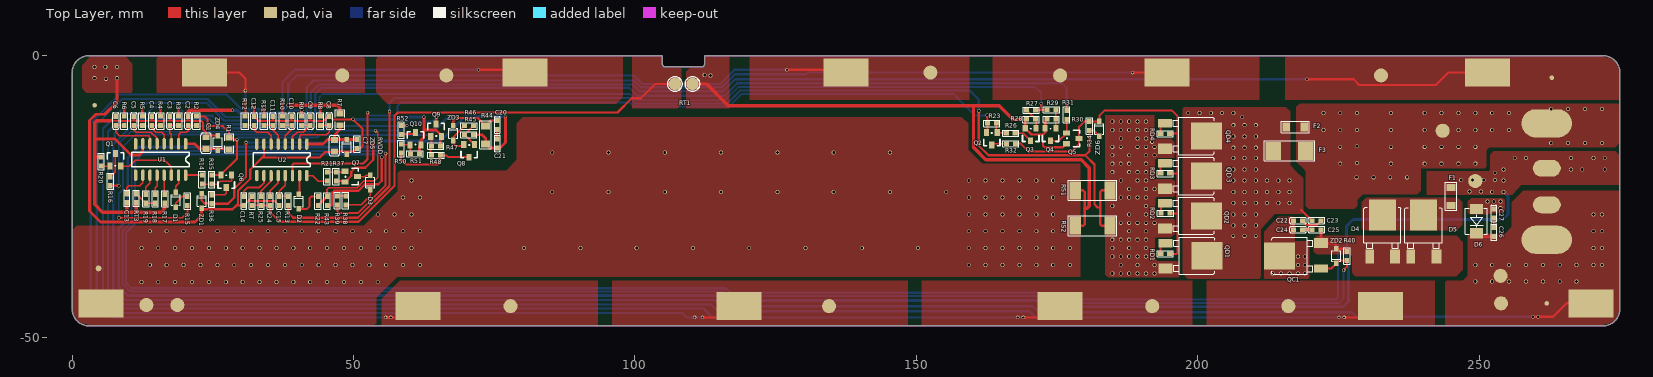
[diagram p0: Top Layer view]
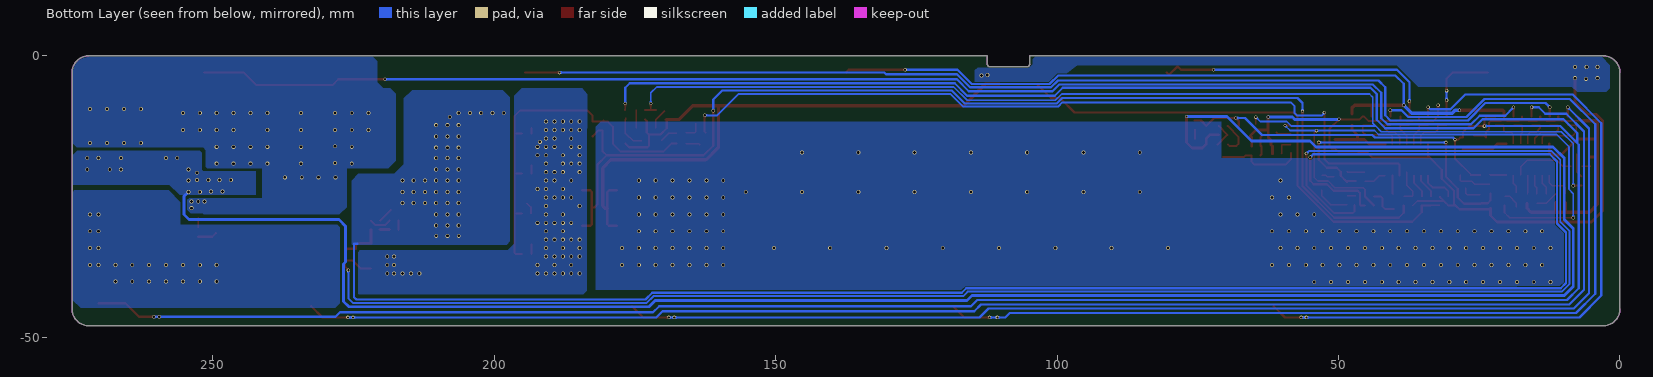
[diagram p1: Bottom Layer view, seen from below]
# Altium PCB MISC86331.PcbDoc
Units mm, origin at the board's own origin, x right, y up, seen from the top; angles counter-clockwise.
Board outline 275 x 48 mm, 2 copper layers (Top Layer, Bottom Layer); 113 components, 80 nets, 305 pads, 410 vias.

## Layer stack, top to bottom (the 12.6 mil dielectric is the usual default, probably not edited)
Top Solder: solder mask 0.0102, Solder Resist, Dk 3.5
Top Layer: signal copper 0.0356
Dielectric 1: dielectric 0.32, FR-4, Dk 4.8
Bottom Layer: signal copper 0.0356
Bottom Solder: solder mask 0.0102, Solder Resist, Dk 3.5

## Board outline
0,-45 0,-3 cw(c3,-3) 3,0 104.875,0 104.875,-1.5 ccw(c105.375,-1.5) 105.375,-2 111.875,-2 ccw(c111.875,-1.5) 112.375,-1.5 112.375,0 272,0 cw(c272,-3) 275,-3 275,-45 cw(c272,-45) 272,-48 3,-48 cw(c3,-45)

## Design rules (kind name [scope] priority, off if disabled: settings)
Clearance "Stitching CS" [IsStitchingVia and InNet('CS') vs (IsVia and (Not IsStitchingVia)) Or IsPad] p1: gap=0.127 ignorepadtopadclearanceinfootprint=FALSE
Clearance [All] p2: gap=0.2 ignorepadtopadclearanceinfootprint=FALSE
ComponentClearance [All] p1: gap=0.2 collisioncheckmode=3 verticalgap=0.254 showdistances=FALSE
PolygonConnect [All] p1: connectstyle=Direct reliefconductorwidth=0.254 reliefentries=4 polygonreliefangle="90 Angle" airgapwidth=0.254
RoutingVias [All] p1: holewidth=0.4 width=0.6 viastyle="Through Hole" minholewidth=0.4 minwidth=0.6 maxholewidth=0.4 maxwidth=0.6
SolderMaskExpansion [All] p1: expansion=0.102 istentingtop=FALSE
Width [All] p1: maxlimit=1 minlimit=0.2 preferedwidth=0.25
29 further rules are at their usual default settings.

## Components (designator, comment, footprint, x,y, rotation, side; value= is the part's Value field where it differs from the comment)
C1 "1uF" CAP0805 23.8,-15.517 r90 top
C2 "0.1uF" C0603A 20.601,-11.58 r180 top
C3 "0.1uF" C0603A 17.388,-11.58 r180 top
C4 "0.1uF" C0603A 14.175,-11.58 r180 top
C5 "0.1uF" C0603A 10.963,-11.58 r180 top
C6 "0.1uF" C0603A 7.75,-11.58 r180 top
C7 "1uF" CAP0805 46.6,-16.016 r270 top
C8 "0.1uF" C0603A 45.68,-11.58 r180 top
C9 "0.1uF" C0603A 42.341,-11.58 r180 top
C10 "0.1uF" C0603A 39.003,-11.58 r180 top
C11 "0.1uF" C0603A 35.665,-11.58 r180 top
C12 "0.1uF" C0603A 32.327,-11.58 r180 top
C13 "0.1uF" C0603A 9.718,-25.324 r0 top
C14 "0.1uF" C0603A 30.5,-25.8 r0 top
C15 "0.1uF" C0603A 36.8,-25.8 r180 top
C20 "0.1uf" C0603A 75.535,-12.323 r0 top
C21 "0.1uf" C0603A 75.535,-15.598 r0 top
C22 "0.1uF" C0603A 217.8,-29.3 r270 top
C23 "0.1uF" C0603A 221.1,-29.3 r90 top
C24 "0.1uF" C0603A 217.8,-30.9 r270 top
C25 "0.1uF" C0603A 221.1,-30.9 r270 top
C26 "0.1uF" C0603A 252.583,-31.354 r0 top
C27 "0.1uF" C0603A 252.583,-28.016 r0 top
D1 "1N4148" SOD323 18.4,-25.608 r90 top
D2 "1N4148" SOD323 40.3,-25.902 r90 top
D3 "1N4148" SOD323 53.016,-22.516 r270 top
D4 "SS510" TO-252-A 230.586,-35.481 r0 top
D5 "SS510" TO-252-A 237.9,-35.5 r0 top
D6 "RS2M" SMB-1 249.483,-29.379 r90 top
F1 "5A" R1206 245,-25 r90 top
F2 "30A" R1206 217.322,-12.65 r0 top
F3 "NC" 2410 213.396,-16.926 r0 top
Q1 "MMBT5401" SOT-23-3 7.7,-18.5 r0 top
Q2 "BSS84" SOT-23-3 163.409,-14.767 r180 top
Q3 "MMBT5551" SOT-23-3 170.31,-14.01 r180 top
Q4 "MMBT5551" SOT-23-3 173.836,-14.01 r180 top
Q5 "MMBT5551" SOT-23-3 177.8,-14.7 r270 top
Q6 "MMBT5401" SOT-23-3 27.4,-22.303 r180 top
Q7 "MMBT5401" SOT-23-3 49.616,-21.472 r270 top
Q8 "MMBT5401" SOT-23-3 70.547,-16.907 r180 top
Q9 "MMBT5551" SOT-23-3 64.668,-13.237 r0 top
Q10 "MMBT5551" SOT-23-3 61.017,-14.746 r0 top
QC1 "NMOS" TO-252-A 221.711,-37.784 r90 top
QD1 "NMOS" TO-252-A 194.467,-33.327 r270 top
QD2 "NMOS" TO-252-A 194.387,-26.237 r270 top
QD3 "NMOS" TO-252-A 194.387,-19.147 r270 top
QD4 "NMOS" TO-252-A 194.387,-12.058 r270 top
R1 "1K" RES0805 27.9,-14.568 r270 top
R2 "1K" RES0603 22.119,-11.581 r0 top
R3 "1K" RES0603 18.906,-11.581 r0 top
R4 "1K" RES0603 15.693,-11.581 r0 top
R5 "1K" RES0603 12.481,-11.581 r0 top
R6 "1K" RES0603 9.268,-11.581 r0 top
R7 "1K" RES0805 47.6,-10.313 r270 top
R8 "1K" RES0603 44.099,-11.581 r0 top
R9 "1K" RES0603 40.761,-11.581 r0 top
R10 "1K" RES0603 37.423,-11.581 r0 top
R11 "1K" RES0603 34.084,-11.581 r180 top
R12 "1K" RES0603 30.746,-11.581 r0 top
R13 "1K" R0603A 38.4,-25.8 r0 top
R14 "5.1M" R0603A 23.1,-22 r0 top
R15 "51K" R0603A 20.5,-25.8 r0 top
R16 "5.1M" R0603A 6.8,-22.3 r180 top
R17 "1K" R0603A 16.505,-25.416 r0 top
R18 "22K" R0603A 14.78,-25.416 r0 top
R19 "35K" R0603A 13.13,-25.416 r0 top
R20 "2M" R0603A 5.2,-18.8 r0 top
R21 "5.1M" R0603A 45.316,-21.472 r180 top
R22 "100K" R0603A 43.7,-25.8 r0 top
R23 "2M" R0603A 163.409,-12.039 r90 top
R24 "22K" R0603A 35.2,-25.8 r0 top
R25 "35K" R0603A 33.6,-25.8 r0 top
R26 "1M" R0603A 166.772,-13.764 r90 top
R27 "1M" R0603A 170.4,-9.7 r90 top
R28 "1M" R0603A 170.38,-11.326 r90 top
R29 "1M" R0603A 174.007,-9.614 r90 top
R30 "1M" R0603A 173.98,-11.326 r90 top
R31 "2M" R0603A 176.7,-10.5 r180 top
R32 "1K" R0603A 166.78,-15.626 r270 top
R34 "5.1M" R0603A 180.75,-12.5 r180 top
R35 "1M" R0603A 24.8,-22 r180 top
R36 "2M" R0603A 24.8,-25.5 r0 top
R37 "1M" R0603A 46.916,-21.472 r0 top
R38 "1M" R0603A 48.6,-25.75 r180 top
R39 "1M" R0603A 47.125,-25.75 r180 top
R40 "3M" R0603A 226.5,-35.6 r0 top
R43 "100K" R0603A 45.3,-25.8 r180 top
R44 "47K/1206" R1206 73.485,-14.073 r90 top
R45 "1M" R0603A 70.485,-14.048 r90 top
R46 "51K" R0603A 70.51,-12.473 r90 top
R47 "100K" R0603A 64.622,-16.065 r90 top
R48 "1M" R0603A 64.68,-17.703 r90 top
R50 "1M" R0603A 58.455,-16.505 r180 top
R51 "100K" R0603A 60.93,-17.405 r90 top
R52 "1K" R0603A 58.467,-13.226 r0 top
RD1 "47R" R0603A 194.217,-35.202 r90 top
RD2 "47R" R0603A 194.292,-28.002 r90 top
RD3 "47R" R0603A 194.217,-20.927 r90 top
RD4 "47R" R0603A 194.217,-13.852 r90 top
RS1 "R0015" 2512 181.267,-23.91 r90 top
RS2 "NC" 2512 181.267,-30.21 r90 top
RT "10K" R0603A 32,-25.8 r180 top
RT1 "103AT" WK 108.6,-5 r180 top
RT3 "10K" R0603A 11.418,-25.324 r0 top
RVDD "5.1M" R0603A 50.6,-15.7 r180 top
U1 "CW1053" SO-16 20.189,-15.636 r180 top
U2 "CW1053" SO-16 41.709,-15.695 r180 top
ZD1 "24V" SOD323 23,-25.8 r90 top
ZD2 "15V" SOD323 224.6,-35.6 r270 top
ZD3 "15V" SOD323 67.735,-13.773 r90 top
ZD4 "24V" SOD323 25.9,-15.5 r270 top
ZD5 "24V" SOD323 48.8,-16.2 r90 top
ZD6 "15V" SOD323 182.5,-13 r90 top

## Footprints (in the part's own frame and the unit in brackets; to place one, negate y for a bottom-side part, rotate by r counter-clockwise, add the part's x,y. Pads: shape width x height; smd on the part's side, far side on the other; paste and mask are expansions set on the pad)
2410 [mm]
  rect 2.8x3.15 smd: 1(0.001,0.001) 2(5.8,0)
  silkscreen extent -1.57,-1.78 7.4,1.78
2512 [mm]
  rect 3.2x2 smd: 1(0,3.05) 2(0,-3.15)
  silkscreen extent -1.8,-4.33 1.8,4.25
C0603A [mm]
  rect 0.8x0.9 smd: 1(0,0.8) 2(0,-0.8)
  silkscreen extent -0.56,-1.45 0.56,1.45
CAP0805 [mil]
  rect 43.31x50 smd: 1(-40,0)
  rect 40x50 smd: 2(40,0)
  silkscreen extent -73,-36 71,36, body extent -39,-25 39,25, height 35
R0603A [mm]
  rect 0.8x0.9 smd: 1(0,0.8) 2(0,-0.8)
  silkscreen extent -0.56,-1.45 0.56,1.45
R1206 [mm]
  rect 1.3x1.6 smd: 1(-1.6,0) 2(1.6,0)
  silkscreen extent -2.47,-1 2.47,1.02
RES0603 [mm] "CAP0402"
  rect 0.88x0.83 smd mask+0: 1(0,0.81) 2(0,-0.81)
  silkscreen extent -0.65,-1.45 0.65,1.45, body extent -0.4,-0.83 0.4,0.77, height 0.3
RES0805 [mil]
  rect 40x50 smd: 1(0,0) 2(80,0)
  silkscreen extent -28,-32 107,32, body extent 1,-25 79,24, height 4
SMB-1 [mm]
  rect 1.8x2.3 smd: 1(2.175,0) 2(-2.175,0)
  silkscreen extent -2.3,-1.95 2.3,1.95
SO-16 [mil]
  oval 24x80 smd: 1(0.36,0.36) 2(50.36,0.36) 3(100.36,0.36) 4(150.36,0.36) 5(200.36,0.36) 6(250.36,0.36) 7(300.36,0.36) 8(350.35,0.35) 9(350.35,220.35) 10(300.36,220.36) 11(250.36,220.36) 12(200.36,220.36) 13(150.36,220.36) 14(100.36,220.36) 15(50.36,220.36) 16(0.36,220.36)
  silkscreen extent -25,60 376,160
SOD323 [mm]
  rect 1x0.8 smd: 1(-1.3,0) 2(1.3,0)
  silkscreen extent -0.92,-0.8 0.93,0.8
SOT-23-3 [mil]
  rect 36x47.24 smd: 1(-37.5,-43.94) 2(37.5,-43.94) 3(0.5,43.94)
  silkscreen extent -58,-41 58,49
TO-252-A [mm]
  rect 1.5x2.5 smd: 1(-0.026,-0.189)
  rect 1.8x2.5 smd: 2(4.484,-0.189)
  rect 4.8x5.5 smd: 3(2.214,7.181)
  silkscreen extent -1.09,1.26 5.51,8.53, body extent -0.95,-0.35 5.35,9.65, height 2.5
WK [mm]
  round 2.2 smd: 1(-1.625,0.025) 2(1.5,0.025)
  silkscreen extent -2.92,-1.27 2.8,1.32

## Part data
C1 C2 C3 C4 C5 C6 C7 C8 C9 C10 C11 C12 C13 C14 C15 C20 C21 C22 C23 C24 C25 C26 C27: library part CAP, "CAP"
D1 D2 D3 D6: library part DIODE, "DIODE"
D4 D5: library part MBR10100DCT, "SMD dual common-cathode diode"
F1 F2 F3: library part FUSE
Q1 Q6 Q7 Q8: library part PNP, "PNP Bipolar Transistor"
Q2: library part PMOS
Q3 Q4 Q5 Q9 Q10: library part NPN, "NPN Bipolar Transistor"
R1 R2 R3 R4 R5 R6 R7 R8 R9 R10 R11 R12 R13 R14 R15 R16 R17 R18 R19 R20 R21 R22 R23 R24 R25 R26 R27 R28 R29 R30 R31 R32 R34 R35 R36 R37 R38 R39 R40 R43 R44 R45 R46 R47 R48 R50 R51 R52 RD1 RD2 RD3 RD4 RS1 RS2 RT RVDD: library part RES1, "RES"
RT1 RT3: library part RES2, "RES"
ZD1 ZD2 ZD3 ZD4 ZD5 ZD6: library part "D Zener", "Zener Diode"

## Free pads (board coordinates)
  round 1 smd: 1(4.7,-37.8)
  round 2.5 smd: 1(13.2,-44.3) 1(18.7,-44.3) 1(48,-3.5) 1(66.5,-3.5) 1(77.9,-44.5) 1(134.5,-44.5) 1(152.5,-3) 1(175.551,-3.5) 1(191.909,-44.5) 1(216.091,-44.5) 1(232.551,-3.5) 1(243.5,-13.332) 1(249.3,-22.273) 1(253.8,-39.1) 1(253.891,-44)
  rect 8x5 smd mask+0: 2(251.5,-3) 3(194.5,-3) 4(137.5,-3) 5(80.5,-3) 6(23.5,-3) 7(5.1,-44) 8(61.491,-44.5) 9(118.5,-44.5) 10(175.5,-44.5) 11(232.5,-44.5) 12(269.9,-44)
  oval 9x5 smd mask+0: 13(262,-32.703) 14(262,-12.016)
  oval 5x3 smd mask+0: 15(262,-20) 16(262,-26.5)
  round 0.8 smd: 600(4,-8.8) 600(262,-44) 600(262.9,-3.9)

## Via types
v1: diameter 0.7, hole 0.5, Top Layer to Bottom Layer, tented both sides, 362 vias
v2: diameter 0.6, hole 0.4, Top Layer to Bottom Layer, tented both sides, 48 vias

## Nets (pads, with @x,y where several pads share a name; then routed paths per layer and width w, separated by ;. In a path a pad name is that pad's centre, name@x,y a point inside that pad or via, vN(x,y) a via of type N, cw(c..) or ccw(c..) an arc to the next point about the centre after c; other vN are vias at no path point)
B1: pad.1@48,-3.5 pad.6 R12.1 | length 14.5
  Top Layer w0.4: pad.6 29.7,-3 30.8,-4.1 v2(30.8,-6.2) ; R12.1 30.8,-10.717 v2(30.8,-7.9)
  Bottom Layer w0.4: v2(30.8,-7.9) 30.8,-6.3 30.75,-6.25 v2(30.8,-6.2)
B2: pad.1@77.9,-44.5 pad.8 R11.2 | length 127.8
  Top Layer w0.4: R11.2 v2(34.084,-9.171) ; v2(55.7,-46.5) v2(56.6,-46.5) 59.491,-46.5 pad.8
  Bottom Layer w0.4: v2(34.084,-9.171) 33.756,-9.5 30.09,-9.5 27.49,-6.9 8.4,-6.9 3.3,-12 3.3,-42.6 7.2,-46.5 v2(55.7,-46.5) v2(56.6,-46.5)
B3: pad.1@66.5,-3.5 pad.5 R10.1 | length 51.1
  Top Layer w0.4: v2(37.4,-8.1) 37.4,-10.749 R10.1 ; v2(72.2,-2.5) 78,-2.5 78.6,-1.9 80.1,-3.4 pad.5
  Bottom Layer w0.4: v2(37.4,-8.1) 37.4,-4.7 39.6,-2.5 71.6,-2.5 v2(72.2,-2.5)
B4: pad.1@134.5,-44.5 pad.9 R9.1 | length 187.9
  Top Layer w0.4: R9.1 v2@40.761,-9.7 ; v2(112,-46.5) 116.5,-46.5 pad.9
  Bottom Layer w0.4: v2(40.8,-9.7) 38.8,-9.7 37.6,-10.9 27.249,-10.9 24.049,-7.7 8.894,-7.7 4.4,-12.194 4.4,-42.3 7.8,-45.7 108.4,-45.7 109.2,-46.5 v2(112,-46.5)
  other v2: 110.6,-46.5
B5: C1.2 C2.2 C3.2 C4.2 C5.2 C6.2 C13.2 pad.1@152.5,-3 pad.4 R7.1 R8.1 R17.2 R20.1 RT3.2 U1.7 ZD4.1 | length 211.1
  Top Layer w0.35: 6.8,-11.555 8.666,-11.555 8.673,-11.561 10.401,-11.561 10.407,-11.555 11.518,-11.555 11.525,-11.561 13.076,-11.561 13.082,-11.555 14.731,-11.555 14.737,-11.561 16.289,-11.561 16.295,-11.555 16.6,-11.555 ; 16.613,-11.555 17.943,-11.555 17.95,-11.561 20.039,-11.561 20.045,-11.555 20.7,-11.555 ; C2.2 20.601,-11.455 20.7,-11.555 ; ZD4.1 24.101,-14.2 C1.2 23.8,-13.6 23.3,-13.1 23.3,-11.9 22.961,-11.561 21.163,-11.561 21.156,-11.555 20.7,-11.555
  Top Layer w0.4: 6.8,-11.555 7.575,-10.78 C6.2 ; 10.963,-11.53 C5.2 ; C4.2 14.175,-11.505 14.2,-11.53 ; C3.2 17.388,-11.518 17.4,-11.53 ; R8.1 44.099,-8.801 ; v2(127,-2.5) 137,-2.5 pad.4
  Top Layer w0.5: 4,-14.8 7.649,-14.8 10.5,-17.651 11.949,-17.651 12.56,-17.04 U1.7
  Top Layer w0.6: R20.1 4,-18 ; 6.8,-11.555 4.345,-11.555 4,-11.9 4,-14.8 4,-18 ; C13.2 9.718,-27.782 9.7,-27.8 ; RT3.2 11.418,-27.718 11.5,-27.8 ; R17.2 16.505,-27.1 15.805,-27.8 11.5,-27.8 ; C2.2 20.601,-9.899 20.8,-9.7 v2(28.5,-9.7) ; v2(38.4,-8.8) 38.401,-8.801 44.099,-8.801 47.13,-8.801 47.6,-9.271 R7.1 ; 4,-18 4,-26.4 5.4,-27.8 9.7,-27.8 ; 9.7,-27.8 11.5,-27.8
  Bottom Layer w0.4: v2(38.4,-8.8) 38.4,-5 39.9,-3.5 99.8,-3.5 101.325,-5.025 115.175,-5.025 117.7,-2.5 v2(127,-2.5)
  Bottom Layer w0.6: v2(28.5,-9.7) 29.3,-9.7 29.8,-10.2 37,-10.2 v2(38.4,-8.8)
B6: pad.1@191.909,-44.5 pad.10 R6.1 | length 208.8
  Top Layer w0.4: R6.1 v2(9.268,-9.171) ; v2(169,-46.5) 173.5,-46.5 pad.10
  Bottom Layer w0.4: v2(9.268,-9.171) 5.5,-12.939 5.5,-42.2 8.2,-44.9 112.2,-44.9 113.8,-46.5 v2(169,-46.5)
  other v2: 168,-46.5
B7: pad.1@175.551,-3.5 pad.3 R5.1 | length 192.7
  Top Layer w0.4: R5.1@12.442,-10.733 R5.1 v2(12.481,-9.171) ; v2(188.4,-3) pad.3
  Bottom Layer w0.4: v2(12.481,-9.171) 13.237,-8.415 23.915,-8.415 27,-11.5 40.8,-11.5 41.7,-10.6 41.7,-5.6 42.9,-4.4 99.851,-4.4 101.076,-5.625 115.475,-5.625 117.8,-3.3 130.4,-3.3 130.7,-3 v2(188.4,-3)
B8: pad.1@216.091,-44.5 pad.11 R4.1 | length 269.8
  Top Layer w0.4: R4.1 v2(15.693,-9.171) ; v2(226,-46.5) 230.5,-46.5 pad.11
  Bottom Layer w0.4: v2(15.693,-9.171) 14.429,-9.171 13.27,-10.33 9.545,-10.33 6.4,-13.475 6.4,-41.6 9,-44.2 113.5,-44.2 114.7,-45.4 170.1,-45.4 171.2,-46.5 v2(226,-46.5)
  other v2: 225.1,-46.5
B9: pad.1@232.551,-3.5 pad.2 pad.600@262.9,-3.9 R3.1 | length 243.7
  Top Layer w0.4: R3.1 v2(18.906,-9.171) ; v2(219.4,-4.2) 227.7,-4.2 228.7,-5.2 241.9,-5.2 242.3,-5.2 244.5,-3 pad.2
  Bottom Layer w0.4: v2(18.906,-9.171) 20.389,-10.655 24.916,-10.655 26.461,-12.2 41.3,-12.2 42.4,-11.1 42.4,-6.6 43.9,-5.1 99.6,-5.1 100.8,-6.3 115.7,-6.3 117.8,-4.2 v2(219.4,-4.2)
B+: C20.1 C26.2 D6.2 pad.1@253.8,-39.1 pad.1@253.891,-44 pad.12 pad.13 pad.16 pad.600@262,-44 Q6.2 R1.1 R2.1 R31.2 R35.2 R44.2 ZD3.2 | length 568
  Top Layer w0.3: R31.2 176.8,-9.6 176.7,-9.5 v2(176.7,-8.5)
  Top Layer w0.35: R2.1 23.571,-10.771 24.081,-11.281 v2(24.081,-12.5) 26.8,-12.5 27.9,-13.6 R1.1 28.381,-14.568 28.713,-14.9 v2(29.3,-14.9) 29.3,-18.334 Q6.2 26.434,-21.2 R35.2 ; Q6.2@26.448,-21.284 Q6.2@26.502,-21.229
  Top Layer w0.4: ZD3.2 67.735,-11.584 v2(68.242,-11.076) 72.088,-11.076 R44.2 74.435,-11.523 C20.1 ; D6.2 250.083,-32.154 C26.2 ; v2(259.5,-46.4) v2(260.5,-46.4) 263.1,-46.4 265.5,-44 pad.12 pad.12@270.3,-44
  Bottom Layer w0.4: v2@24.1,-12.5 v2(24.081,-12.5) 10.622,-12.5 7.6,-15.522 ; v2(29.3,-14.9) 29.65,-14.55 43.535,-14.55 43.985,-14.1 63.6,-14.1 66.624,-11.076 v2(68.242,-11.076) ; v2(176.7,-8.5) 176.7,-5.7 175.9,-4.9 118.2,-4.9 116,-7.1 100.4,-7.1 99,-5.7 44.3,-5.7 43.2,-6.8 43.2,-11.4 41.7,-12.9 26.025,-12.9 24.425,-11.3 10.025,-11.3 7.6,-13.725 7.6,-15.522 ; v2(260.5,-46.4) v2(259.5,-46.4) 228.2,-46.4 227.4,-45.6 171.8,-45.6 170.7,-44.5 115.3,-44.5 114.2,-43.4 9.4,-43.4 7.3,-41.3 7.3,-15.822 7.6,-15.522
  other v1: 249.309,-40.09 252.309,-40.09 255.309,-40.09 258.309,-40.09 261.309,-40.09 264.309,-40.09 267.309,-40.09 249.309,-37.19 252.309,-37.19 255.309,-37.19 258.309,-37.19 261.309,-37.19 264.309,-37.19 267.309,-37.19 270.309,-37.19 271.809,-37.19 270.309,-34.19 271.809,-34.19 270.309,-31.19 271.809,-31.19 270.309,-28.19 271.809,-28.19
B-: C7.2 C8.2 C9.2 C10.2 C11.2 C12.2 C14.2 C15.1 pad.1@4.7,-37.8 pad.1@13.2,-44.3 pad.1@18.7,-44.3 pad.7 Q3.2 Q4.2 Q5.2 Q9.2 Q10.2 R28.1 R30.1 R47.2 R51.2 RS1.1 RS2.1 RT1.1 RT.2 RVDD.1 U2.7 ZD1.1 ZD5.1 | length 273.1
  Top Layer w0.3: 31.075,-26.025 31.3,-25.8 36,-25.8 C15.1
  Top Layer w0.35: ZD1.1 ZD1.1@23.2,-27.3 ; C14.2 31.075,-26.025 ; 31.3,-25.8 32,-25.1 RT.2 ; C12.2 33.108,-11.561 34.68,-11.561 34.686,-11.555 35.6,-11.555 ; C11.2 35.665,-11.49 35.6,-11.555 ; C10.2 39.003,-11.452 38.9,-11.555 ; C9.2 42.341,-11.513 42.3,-11.555 ; C7.2@46.537,-17.095 C7.2 50.068,-17.032 RVDD.1 51.2,-16.5 51.6,-16.1 51.6,-13 v2(49.9,-11.3) 46.251,-11.3 46.226,-11.326 C8.2 45.476,-10.78 44.694,-11.561 42.903,-11.561 42.897,-11.555 42.3,-11.555 ; 35.6,-11.555 36.22,-11.555 36.821,-11.555 36.827,-11.561 38.018,-11.561 38.024,-11.555 38.9,-11.555 ; 38.9,-11.555 39.559,-11.555 39.565,-11.561 41.356,-11.561 41.363,-11.555 42.3,-11.555
  Top Layer w0.4: ZD1.1@23.2,-27.3 28.5,-27.3 29.2,-26.6 ; C14.2 29.2,-26.6 ; v2(32.3,-8.8) 32.3,-10.753 C12.2 ; U2.7 34.08,-17.82 33.8,-18.1 ; C7.2@46.537,-17.095 45,-17.095 43.995,-18.1 33.8,-18.1 ; R28.1 169.358,-11.548 Q3.2 170.463,-14 172.486,-14 ; R30.1 172.883,-11.622 Q4.2 172.883,-13.602 172.486,-14 ; Q5.2 176.062,-16.275 172.775,-16.275 172.486,-15.986 172.486,-14 ; RS2.1 179.64,-30.21 179.9,-29.95 179.9,-27.087 179.9,-24.225 179.585,-23.91 RS1.1 ; 29.2,-26.6 29.5,-26.3 29.5,-24 31.65,-21.85 31.65,-20.25 33.8,-18.1
  Top Layer w0.5: v1(8,-4) 8,-8.2 5.8,-10.4 4.232,-10.4 3.1,-11.532 3.1,-27.6 5.05,-29.55 21.85,-29.55 23,-28.4 ZD1.1 ; R51.2 61.73,-16.102 Q10.2 61.97,-15.03 62.478,-14.522 62.478,-13.2 ; v2(62.5,-10.9) 62.5,-13.178 62.478,-13.2 ; R47.2 65.422,-14.551 Q9.2 65.62,-14.152 64.668,-13.2 62.478,-13.2
  Top Layer w0.6: RT1.1 112.725,-5.025 116.6,-8.9 160.1,-8.9 ; R28.1@169.358,-11.326 167.126,-11.326 164.7,-8.9 160.1,-8.9 ; 179.9,-27.087 180.363,-27.087 180.748,-26.702 180.748,-19.948 179.3,-18.5 162.367,-18.5 160.15,-16.283 160.15,-8.95 160.1,-8.9
  Bottom Layer w0.5: v2(49.9,-11.3) 49.926,-11.326 57.774,-11.326 58.2,-10.9 v2(62.5,-10.9)
  other v1: 12.309,-40.19 15.309,-40.19 18.309,-40.19 21.309,-40.19 24.309,-40.19 27.309,-40.19 30.309,-40.19 33.309,-40.19 36.309,-40.19 39.309,-40.19 42.309,-40.19 45.309,-40.19 48.309,-40.19 51.309,-40.19 54.309,-40.19 13.809,-37.19 16.809,-37.19 19.809,-37.19 22.809,-37.19 25.809,-37.19 28.809,-37.19 31.809,-37.19 34.809,-37.19 37.809,-37.19 40.809,-37.19 43.809,-37.19 46.809,-37.19 49.809,-37.19 52.809,-37.19 55.809,-37.19 58.809,-37.19 61.809,-37.19 159.309,-37.19 162.309,-37.19 165.309,-37.19 168.309,-37.19 171.309,-37.19 174.309,-37.19 177.309,-37.19 12.309,-34.19 15.309,-34.19 18.309,-34.19 21.309,-34.19 24.309,-34.19 27.309,-34.19 30.309,-34.19 33.309,-34.19 36.309,-34.19 39.309,-34.19 42.309,-34.19 45.309,-34.19 48.309,-34.19 51.309,-34.19 54.309,-34.19 57.309,-34.19 60.309,-34.19 80.309,-34.19 90.309,-34.19 100.309,-34.19 110.309,-34.19 120.309,-34.19 130.309,-34.19 140.309,-34.19 150.309,-34.19 159.309,-34.19 162.309,-34.19 165.309,-34.19 168.309,-34.19 171.309,-34.19 174.309,-34.19 177.309,-34.19 13.809,-31.19 16.809,-31.19 19.809,-31.19 22.809,-31.19 25.809,-31.19 28.809,-31.19 31.809,-31.19 34.809,-31.19 37.809,-31.19 40.809,-31.19 43.809,-31.19 46.809,-31.19 49.809,-31.19 52.809,-31.19 55.809,-31.19 58.809,-31.19 61.809,-31.19 159.309,-31.19 162.309,-31.19 165.309,-31.19 168.309,-31.19 171.309,-31.19 174.309,-31.19 54.309,-28.19 57.309,-28.19 60.309,-28.19 159.309,-28.19 162.309,-28.19 165.309,-28.19 168.309,-28.19 171.309,-28.19 174.309,-28.19 58.809,-25.19 61.809,-25.19 159.309,-25.19 162.309,-25.19 165.309,-25.19 168.309,-25.19 171.309,-25.19 174.309,-25.19 85.309,-24.19 95.309,-24.19 105.309,-24.19 115.309,-24.19 125.309,-24.19 135.309,-24.19 145.309,-24.19 155.309,-24.19 60.309,-22.19 159.309,-22.19 162.309,-22.19 165.309,-22.19 168.309,-22.19 171.309,-22.19 174.309,-22.19 85.309,-17.19 95.309,-17.19 105.309,-17.19 115.309,-17.19 125.309,-17.19 135.309,-17.19 145.309,-17.19 6,-4.1 4,-4 113.4,-3.5 112.391,-3.441 4,-2 5.9,-2 8,-2
C-: C21.2 F1.2 pad.1@249.3,-22.273 pad.15 R44.1 R45.2 | length 373.6
  Top Layer w0.5: R45.2 72.848,-14.048 73.485,-14.685 R44.1 74.21,-16.398 C21.2 76,-16.398 77,-15.398 v2(77,-10.8)
  Bottom Layer w0.5: v2(77,-10.8) 69.8,-10.8 65.474,-15.126 55.074,-15.126 54,-16.2 11.9,-16.2 9.9,-18.2 9.9,-29.1 8.3,-30.7 8.3,-41 9.9,-42.6 115.1,-42.6 116,-43.5 171.4,-43.5 172.5,-44.6 225.8,-44.6 226.75,-43.65 226.75,-37 226.4,-36.65 226.4,-30.3 227.6,-29.1 254.2,-29.1 255.1,-28.2 255.1,-24.98 v1(254.309,-24.19)
  other v1: 252.309,-24.19 248.3,-24.1 250.3,-24.1 254.309,-22.19 246.8,-22.1 248.8,-22.1 250.8,-22.1 252.8,-22.1 252.809,-20.79 254.309,-20.19 266.309,-20.19 268.309,-20.19 272.309,-20.19 256.309,-18.19 258.309,-18.19 266.309,-18.19 270.309,-18.19 272.309,-18.19
CO1: Q6.1 R14.2 R35.1 | length 6.7
  Top Layer w0.25: R14.2 R35.1 ; R35.1@24.953,-22.952 R35.1 ; Q6.1 28.353,-22.147 28.2,-22.3 26.3,-22.3 25.8,-22.8 R35.1
CO2: Q7.1 R21.2 R37.1 | length 3.2
  Top Layer w0.25: R21.2 R37.1 48.348,-20.672 Q7.1
CS: C22.2 C24.2 QC1.3 QD1.2 QD2.2 QD3.2 QD4.2 R13.2 R34.1 RS1.2 RS2.2 ZD6.1 | length 200.3
  Top Layer w0.4: R13.2 38.4,-27.9 39.3,-28.8 50.751,-28.8 56.4,-23.151 v2(56.4,-9.9) ; v2(161.1,-9.8) 161.1,-16 162.803,-17.703 180.003,-17.703 ; ZD6.1 181.5,-13.3 R34.1 180.75,-16.956 180.003,-17.703 ; RS2.2 182.91,-30.21 182.65,-29.95 182.65,-26.95 ; RS1.2 182.94,-23.91 182.65,-24.2 182.65,-26.95 ; C24.2 C22.2 ; 180.003,-17.703 181.65,-19.35 181.65,-26.4 182.2,-26.95 182.65,-26.95
  Bottom Layer w0.4: v2(56.4,-9.9) 56.4,-8.4 57.3,-7.5 99.092,-7.5 100.072,-8.48 116.42,-8.48 118.7,-6.2 159.5,-6.2 161.1,-7.8 v2(161.1,-9.8)
  other v1: 184.809,-38.69 186.309,-38.69 187.809,-38.69 189.309,-38.69 190.809,-38.69 192.309,-38.69 213.309,-38.69 214.809,-38.69 216.309,-38.69 217.809,-38.69 219.009,-38.671 186.309,-37.19 189.309,-37.19 192.309,-37.19 217.809,-37.19 219.009,-37.171 184.809,-35.69 186.309,-35.69 187.809,-35.69 189.309,-35.69 190.809,-35.69 217.809,-35.69 219.009,-35.671 184.809,-34.19 187.809,-34.19 190.809,-34.19 184.809,-32.69 186.309,-32.69 187.809,-32.69 189.309,-32.69 190.809,-32.69 187.809,-31.19 190.809,-31.19 186.309,-29.69 187.809,-29.69 189.309,-29.69 190.809,-29.69 192.309,-29.69 187.809,-28.19 190.809,-28.19 184.809,-26.69 190.809,-26.69 186.309,-25.19 187.809,-25.19 189.309,-25.19 190.809,-25.19 187.809,-23.69 190.809,-23.69 192.309,-23.69 186.309,-22.19 189.309,-22.19 190.809,-22.19 184.809,-20.69 187.809,-20.69 189.309,-20.69 190.809,-20.69 184.809,-19.19 186.309,-19.19 187.809,-19.19 190.809,-19.19 184.809,-17.69 187.809,-17.69 190.809,-17.69 192.309,-17.69 184.809,-16.19 186.309,-16.19 189.309,-16.19 190.809,-16.19 192.309,-16.19 191.9,-15.3 186.309,-14.69 189.309,-14.69 190.809,-14.69 184.809,-13.19 186.309,-13.19 187.809,-13.19 189.309,-13.19 190.809,-13.19 184.809,-11.69 186.309,-11.69 187.809,-11.69 189.309,-11.69 190.809,-11.69
DO1: Q9.3 R16.1 R27.2 R29.1 | length 209.2
  Top Layer w0.3: Q9.3 v2(64.68,-10.906) ; v2(172.2,-8.5) 172.2,-9.544 172.235,-9.579 ; R29.1@173.1,-9.614 R29.1@173.135,-9.579
  Top Layer w0.35: R16.1 v2@8.25,-23.1 ; R27.2@171.262,-9.614 173.1,-9.614 R29.1
  Bottom Layer w0.3: v2(8.3,-23.1) 8.3,-15.6 10.4,-13.5 42.4,-13.5 43.4,-12.5 ; v2(64.68,-10.906) 63.887,-11.7 59.193,-11.7 58.393,-12.5 43.4,-12.5 ; v2(172.2,-8.5) 172.2,-6.6 171.15,-5.55 118.35,-5.55 115.97,-7.93 100.3,-7.93 99.17,-6.8 44.5,-6.8 43.9,-7.4 43.9,-12 43.4,-12.5
NetC1_1: C1.1 R1.2 U1.1 ZD4.2 | length 8.1
  Top Layer w0.5: U1.1 21.745,-15.645 22.633,-16.533 C1.1 27.833,-16.533 R1.2
NetC2_1: C2.1 R2.2 U1.2 | length 6
  Top Layer w0.25: U1.2 18.91,-14.07 19.34,-13.64 20.26,-13.64 20.601,-13.299 C2.1 20.612,-12.391 R2.2
NetC3_1: C3.1 R3.2 U1.3 | length 4.9
  Top Layer w0.25: U1.3 17.64,-13.964 17.388,-13.712 C3.1 17.4,-12.391 R3.2
NetC4_1: C4.1 R4.2 U1.4 | length 6.3
  Top Layer w0.25: R4.2 15.682,-12.38 C4.1 14.175,-12.84 14.9,-13.565 15.935,-13.565 16.37,-14 U1.4
NetC5_1: C5.1 R5.2 U1.5 | length 8
  Top Layer w0.25: R5.2 12.469,-12.38 C5.1 10.963,-13.195 11.368,-13.6 14,-13.6 15.1,-14.7 U1.5
NetC6_1: C6.1 R6.2 U1.6 | length 10.4
  Top Layer w0.25: R6.2 9.277,-12.4 7.77,-12.4 C6.1 7.75,-13.55 8.4,-14.2 13.584,-14.2 13.83,-14.446 U1.6
NetC7_1: C7.1 R7.2 RVDD.2 U2.1 ZD5.2 | length 12.3
  Top Layer w0.5: U2.1 44.596,-15.704 45.4,-14.9 C7.1@46.6,-14.9 ; C7.1 C7.1@46.6,-14.9 ; R7.2 47.6,-13.1 46.6,-14.1 C7.1@46.6,-14.9 ; RVDD.2 ZD5.2 C7.1@46.6,-14.9
NetC8_1: C8.1 R8.2 U2.2 | length 9.8
  Top Layer w0.25: U2.2 40.43,-14.27 40.615,-14.085 45.179,-14.085 45.68,-13.585 C8.1 45.668,-12.391 R8.2
NetC9_1: C9.1 R9.2 U2.3 | length 6.9
  Top Layer w0.25: U2.3 39.16,-14.44 39.965,-13.635 41.1,-13.635 42.341,-12.394 C9.1 42.33,-12.391 R9.2
NetC10_1: C10.1 R10.2 U2.4 | length 5.4
  Top Layer w0.25: R10.2 37.434,-12.38 C10.1 39.003,-13.097 37.89,-14.21 U2.4
NetC11_1: C11.1 R11.1 U2.5 | length 5.3
  Top Layer w0.25: R11.1 35.653,-12.391 C11.1 35.665,-13.165 36.62,-14.12 U2.5
NetC12_1: C12.1 R12.2 U2.6 | length 7.3
  Top Layer w0.25: R12.2@30.735,-12.38 R12.2 32.315,-12.391 C12.1 32.327,-13.127 32.835,-13.635 34.735,-13.635 35.35,-14.25 U2.6
NetC13_1: C13.1 U1.10 | length 5.6
  Top Layer w0.25: C13.1 9.718,-23.482 10.1,-23.1 12.062,-23.1 12.56,-22.602 U1.10
NetC14_1: C14.1 U2.10 | length 6.4
  Top Layer w0.35: C14.1 30.5,-24.115 31.215,-23.4 33.3,-23.4 34.08,-22.62 U2.10
NetC15_2: C15.2 R13.1 U2.13 | length 6.5
  Top Layer w0.25: U2.13@37.89,-20.6 U2.13 37.89,-23.01 36.8,-24.1 C15.2 R13.1
NetC20_2: C20.2 C21.1 | length 1.7
  Top Layer w0.35: C21.1 C20.2
NetC22_1: C22.1 C23.2 | length 4
  Top Layer w0.4: C22.1 219.4,-30.1 221.1,-30.1 C23.2
NetC23_1: C23.1 F2.1 F3.1 QD1.3 QD2.3 QD3.3 QD4.3 R43.1 | length 313.2
  Top Layer w0.4: R43.1 46.083,-26.6 46.2,-26.483 46.2,-24.4 46.6,-24 50.878,-24 52.055,-22.822 54.399,-22.822 55,-22.222 v2(55,-18.023) ; 218.4,-27.4 C23.1
  Bottom Layer w0.4: v2(55,-18.023) 54.477,-17.5 12.481,-17.5 11.175,-18.806 11.175,-29.825 9.6,-31.4 9.6,-40.387 10.513,-41.3 18.2,-41.3 18.225,-41.325 116.138,-41.325 116.938,-42.125 171.938,-42.125 173.138,-43.325 224.475,-43.325 224.9,-42.9 224.9,-33.4 224.3,-33.4
  other v1: 206.3,-32 208.3,-32 210.3,-32 206.309,-30.19 208.309,-30.19 210.309,-30.19 206.309,-28.19 208.309,-28.19 210.309,-28.19 206.309,-26.19 208.309,-26.19 210.309,-26.19 212.309,-26.19 214.309,-26.19 216.309,-26.19 206.309,-24.19 208.309,-24.19 210.309,-24.19 212.309,-24.19 214.309,-24.19 216.309,-24.19 206.309,-22.19 208.309,-22.19 210.309,-22.19 212.309,-22.19 214.309,-22.19 216.309,-22.19 206.309,-20.19 208.309,-20.19 210.309,-20.19 206.309,-18.19 208.309,-18.19 210.309,-18.19 206.309,-16.345 208.309,-16.345 210.309,-16.345 206.309,-14.345 208.309,-14.345 210.309,-14.345 206.309,-12.345 208.309,-12.345 210.309,-12.345 207.9,-10.9 198.309,-10.19 200.309,-10.19 202.309,-10.19 204.309,-10.19 206.309,-10.19
NetC24_1: C24.1 C25.2 | length 1.7
  Top Layer w0.5: C24.1 C25.2
NetC25_1: C25.1 D4.1 D4.2 D5.1 D5.2 QC1.2 R40.1 ZD2.1 | length 8
  Top Layer w0.4: QC1.2 224.2,-33.3 224.6,-33.7 ZD2.1 226,-34.3 R40.1
  Top Layer w0.6: QC1.2 C25.1
NetC26_1: C26.1 C27.2 | length 1.7
  Top Layer w0.35: C26.1 C27.2
NetD1_1: D1.1 R15.1 | length 3.3
  Top Layer w0.25: D1.1 18.4,-26.2 19.6,-25 R15.1
NetD1_2: D1.2 U1.15 | length 3.3
  Top Layer w0.25: D1.2 18.4,-23.21 18.91,-22.7 U1.15
NetD2_1: D2.1 R22.1 | length 5.4
  Top Layer w0.35: D2.1@40.1,-27.202 D2.1 41.784,-27.202 42.2,-26.786 42.2,-25.3 42.5,-25 R22.1
NetD2_2: D2.2 U2.15 | length 3.4
  Top Layer w0.35: D2.2 40.43,-24.472 U2.15
NetD3_1: D3.1 Q7.3 | length 2.4
  Top Layer w0.25: Q7.3 52.015,-21.485 52.284,-21.216 D3.1
NetD3_2: D3.2 R38.1 | length 6.3
  Top Layer w0.25: R38.1@48.45,-26.508 51.408,-26.508 53.016,-24.9 D3.2
NetD4_3: D4.3 D5.3 F1.1
NetQ1_1: Q1.1 R20.2 | length 1.6
  Top Layer w0.25: R20.2 6.731,-19.6 Q1.1
NetQ1_2: Q1.2 U1.14 | length 11.4
  Top Layer w0.25: Q1.2 10.184,-19.616 11.2,-18.6 16.5,-18.6 17.64,-19.74 U1.14
NetQ1_3: Q1.3 R16.2 | length 4.5
  Top Layer w0.25: R16.2 7.713,-20.587 Q1.3
NetQ2_1: Q2.1 R23.2 R26.1 | length 3.3
  Top Layer w0.25: R23.2 164.209,-13.499 Q2.1 165.86,-13.651 R26.1
NetQ2_2: Q2.2 R23.1 U2.14 | length 141.8
  Top Layer w0.35: U2.14 39.16,-19.39 39.4,-19.15 51.7,-19.15 52.5,-18.35 v2(52.5,-10.1) ; Q2.2 162.609,-13.499 R23.1 v2@162.609,-10.691
  Bottom Layer w0.35: v2(52.5,-10.1) 52.5,-10.2 52.9,-10.6 57.4,-10.6 57.8,-10.2 57.8,-9 58.5,-8.3 99.079,-8.3 99.834,-9.055 116.658,-9.055 118.938,-6.775 156.575,-6.775 160.409,-10.609 160.419,-10.6 v2(162.6,-10.6)
NetQ2_3: Q2.3 R32.2 | length 2.7
  Top Layer w0.25: Q2.3 163.654,-15.626 R32.2
NetQ3_1: Q3.1 R27.1 R28.2 | length 3.7
  Top Layer w0.25: R27.1@169.662,-9.808 R28.2 171.263,-11.408 Q3.1
NetQ3_3: Q3.3 R26.2 | length 3.3
  Top Layer w0.25: R26.2 167.572,-13.819 168.99,-13.819 Q3.3
NetQ4_1: Q4.1 R29.2 R30.2 | length 3.3
  Top Layer w0.25: Q4.1 174.788,-9.632 R29.2
NetQ4_3: Q4.3 Q5.1 R31.1 | length 6.1
  Top Layer w0.25: Q4.3 175.305,-15.126 Q5.1 176.684,-11.344 176.64,-11.3 R31.1@176.64,-11.058
NetQ5_3: Q5.3 R32.1 R34.2 RD1.2 RD2.2 RD3.2 RD4.2 ZD6.2 | length 65.4
  Top Layer w0.35: R32.1 168.526,-15.626 169.932,-17.032 177.537,-17.032 178.916,-15.653 Q5.3 178.916,-12.584 179.8,-11.7 R34.2 ZD6.2 182.5,-10.7 183.475,-9.725 195.371,-9.725 196.425,-10.779 196.425,-13.9 ; R34.2@180.625,-11.525 R34.2@180.775,-11.675 ; RD1.2 196.223,-35.202 196.425,-35 196.425,-27.9 ; RD3.2 196.398,-20.927 196.425,-20.9 ; RD4.2 196.377,-13.852 196.425,-13.9 ; RD2.2 196.323,-28.002 196.425,-27.9 ; 196.425,-27.9 196.425,-20.9 ; 196.425,-20.9 196.425,-13.9
NetQ6_3: Q6.3 R36.1 | length 3.7
  Top Layer w0.25: R36.1 27.124,-24.7 27.387,-24.437 Q6.3
NetQ7_2: Q7.2 R36.2 R37.2 ZD1.2 | length 52.6
  Top Layer w0.4: ZD1.2 23,-25.7 23.5,-26.2 24.7,-26.2 R36.2 27.7,-26.3 28.8,-25.2 28.8,-23.625 30.9,-21.525 v2(30.9,-15.4) ; R37.2 48.348,-22.273 Q7.2 49.6,-21.325 49.6,-20.6 50.3,-19.9 52.1,-19.9 53.5,-18.5 v2(53.5,-15.4)
  Bottom Layer w0.4: v2(30.9,-15.4) v2@53.3,-15.4
NetQ8_1: Q8.1 R45.1 R46.2 | length 4.8
  Top Layer w0.35: R45.1 R45.1@69.735,-14.048 ; R46.2 R45.1@69.735,-14.048 ; Q8.1 69.757,-14.048 R45.1@69.735,-14.048
NetQ8_2: Q8.2 R46.1 ZD3.1 | length 6.1
  Top Layer w0.35: Q8.2 69.36,-16.026 68.142,-16.026 67.735,-15.619 ZD3.1 67.735,-14.448 R46.1
NetQ8_3: Q8.3 R48.2 R50.1 | length 15
  Top Layer w0.35: R50.1 58.455,-18.439 59.342,-19.326 64.942,-19.326 65.48,-18.788 R48.2 66.518,-17.703 66.838,-18.023 Q8.3
NetQ9_1: Q9.1 R47.1 R48.1 | length 3.5
  Top Layer w0.35: R47.1@63.715,-16.065 63.715,-17.538 R48.1 ; Q9.1 63.822,-14.459 R47.1
NetQ10_1: Q10.1 R50.2 R51.1 | length 3.2
  Top Layer w0.25: R50.2 58.612,-15.862 Q10.1 60.065,-17.34 R51.1
NetQ10_3: Q10.3 R52.2 | length 2.6
  Top Layer w0.35: R52.2@58.522,-13.923 60.737,-13.923 Q10.3
NetQC1_1: QC1.1 R39.1 R40.2 ZD2.2 | length 317
  Top Layer w0.35: R39.1 47.125,-27.625 47.475,-27.975 50.763,-27.975 55.7,-23.038 v2(55.7,-17.384) ; ZD2.2@224.49,-37.01 ZD2.2 225.1,-36.4 R40.2 226.5,-37.5 v2(225.9,-38.1)
  Top Layer w0.4: QC1.1 223.69,-37.81 ZD2.2@224.49,-37.01
  Bottom Layer w0.35: v2(55.7,-17.384) 55.216,-16.9 12.2,-16.9 10.6,-18.5 10.6,-29.503 9,-31.103 9,-40.6 10.3,-41.9 115.9,-41.9 116.7,-42.7 171.7,-42.7 172.9,-43.9 225.1,-43.9 225.9,-43.1 v2(225.9,-38.1)
NetQD1_1: QD1.1 RD1.1 | length 1.6
  Top Layer w0.35: RD1.1 QD1.1@193.417,-33.575
NetQD2_1: QD2.1 RD2.1 | length 2.1
  Top Layer w0.35: RD2.1 193.492,-26.917 QD2.1
NetQD3_1: QD3.1 RD3.1 | length 1.4
  Top Layer w0.35: RD3.1 QD3.1@193.417,-19.525
NetQD4_1: QD4.1 RD4.1 | length 1
  Top Layer w0.35: RD4.1 193.417,-12.812
NetR14_1: R14.1 U1.16 | length 3
  Top Layer w0.35: U1.16 22.941,-21.233 R14.1@23.1,-21.075
NetR17_1: R17.1 U1.13 | length 3.4
  Top Layer w0.25: U1.13 16.37,-24.481 R17.1
NetR18_1: R18.1 U1.12 | length 3.5
  Top Layer w0.25: R18.1 14.78,-23.42 15.1,-23.1 U1.12
NetR18_2: R18.2 R19.2 RT3.1 | length 4.2
  Top Layer w0.25: RT3.1 13.11,-26.216 R19.2 R18.2 ; R19.2@13.04,-26.316 R19.2@13.13,-26.226
NetR19_1: R19.1 U1.11 | length 3.7
  Top Layer w0.25: R19.1 13.13,-23.37 13.83,-22.67 U1.11
NetR21_1: R21.1 U2.16 | length 4
  Top Layer w0.25: U2.16 42.74,-21.292 43.72,-22.273 R21.1
NetR24_1: R24.1 U2.12 | length 4.3
  Top Layer w0.35: R24.1 35.2,-24.016 36.62,-22.596 U2.12
NetR24_2: R24.2 R25.2 RT1.2 RT.1 | length 94.4
  Top Layer w0.25: RT.1 R25.2
  Top Layer w0.4: R25.2 R24.2 35.2,-27.8 36.9,-29.5 50.9,-29.5 57.3,-23.1 57.3,-10.7 57.9,-10.1 96.9,-10.1 99.437,-7.563 101.051,-7.563 103.589,-5.025 RT1.2
NetR25_1: R25.1 U2.11 | length 4.4
  Top Layer w0.35: R25.1 33.6,-24 35.35,-22.25 U2.11
NetR38_2: R38.2 R39.2 | length 1.5
  Top Layer w0.25: R39.2@46.9,-24.908 R38.2@48.45,-24.908
P-: C27.1 D6.1 F2.2 F3.2 pad.1@243.5,-13.332 pad.14
  other v1: 253.8,-27.086 251.5,-25.9 252.583,-25.9 253.8,-25.9 228.2,-21.6 231.2,-21.6 234.2,-21.6 237.2,-21.6 225.309,-19.19 234.309,-19.19 240.309,-19.19 243.309,-19.19 246.309,-19.19 249.309,-19.19 228.309,-19.09 225.309,-16.19 234.309,-16.19 240.309,-16.19 243.309,-16.19 246.309,-16.19 249.309,-16.19 228.309,-16.09 262.79,-15.491 265.79,-15.491 268.79,-15.491 271.79,-15.491 222.309,-13.19 225.309,-13.19 228.309,-13.19 234.309,-13.19 240.309,-13.19 246.309,-13.19 249.309,-13.19 252.309,-13.19 255.309,-13.19 222.309,-10.19 225.309,-10.19 228.309,-10.19 234.309,-10.19 240.309,-10.19 243.309,-10.19 246.309,-10.19 249.309,-10.19 252.309,-10.19 255.309,-10.19 262.79,-9.491 265.79,-9.491 268.79,-9.491 271.79,-9.491
VM: R15.2 R22.2 R43.2 R52.1 | length 101.7
  Top Layer w0.3: v2(8.3,-28.8) 8.325,-28.775 19.575,-28.775 20.5,-27.85 R15.2 ; R43.2 45.3,-23.75 45.6,-23.45 50.65,-23.45 51.828,-22.273 53.677,-22.273 54.3,-21.65 54.3,-13.7 v2(53.9,-13.3)
  Top Layer w0.4: R22.2 R43.2 ; R52.1 58.493,-12.4 v2(59.5,-12.4)
  Bottom Layer w0.3: v2(8.3,-28.8) 8.3,-24.5 9.05,-23.75 9.05,-16.15 11.2,-14 42.9,-14 43.6,-13.3 v2(53.9,-13.3) 58.6,-13.3 v2(59.5,-12.4)
pads on no net: U1.8 U1.9 U2.8 U2.9

## Polygon pours and split planes (outlines as drawn)
P- on Top Layer "Top Layer-P- 2" (solid, remove dead copper, pour order 396): 218.7,-20 219.2,-20.5 219.2,-26.686 219.73,-27.216 227.784,-27.216 228.3,-26.7 228.3,-25.6 229.284,-24.616 238.984,-24.616 239.6,-24 239.6,-19.3 219.3,-19.3 218.7,-19.9
NetC25_1 on Top Layer "Top Layer-NetC25_1" (solid, remove dead copper, pour order 394): 246,-32 247.1,-33.1 247.1,-38 245.9,-39.2 228,-39.2 227.4,-38.6 227.4,-35.6 227.1,-35.3 221.1,-35.3 220.6,-34.8 220.6,-32.5 221.1,-32
NetD4_3 on Top Layer "Top Layer-NetD4_2" (solid, remove dead copper, pour order 356): 229.1,-26 229.9,-25.2 246.2,-25.2 247,-26 247,-30 246,-31 229.422,-31 229.1,-30.71 229.1,-29.9
B7 on Top Layer "NONET_L-01_P-001" (solid, pour order 323): 163.575,-7.814 163.575,-0.014 210.639,-0.014 210.9,-0.275 210.9,-7.814
CS on Top Layer "Top Layer-CS" (solid, remove dead copper, pour order 390): 211.8,-31.3 214.3,-28.6 217,-28.6 217.2,-28.8 217.2,-33 219.8,-33 219.8,-39.4 219.6,-39.6 211.8,-39.6
NetC23_1 on Top Layer "Top Layer-NetC23_1" (solid, remove dead copper, pour order 384): 198.259,-39.6 197.3,-38.641 197.3,-9.4 197.529,-9.171 215.671,-9.171 216.4,-9.9 216.4,-19.503 217.497,-20.6 218.7,-21.803 218.7,-27.9 218.5,-28.1 213.668,-28.1 211.2,-30.847 211.2,-39.3 210.9,-39.6
CS on Top Layer "b" (solid, remove dead copper, pour order 378): 196.623,-39.4 196.623,-36.894 196.248,-36.519 192.923,-36.519 192.398,-35.994 192.398,-32.444 192.598,-32.244 195.273,-32.244 195.898,-31.619 195.898,-29.219 195.673,-28.994 192.648,-28.994 192.448,-28.794 192.448,-25.344 192.748,-25.044 195.623,-25.044 195.873,-24.794 195.873,-22.344 195.448,-21.919 192.473,-21.919 192.348,-21.794 192.348,-18.544 192.64,-18.252 195.673,-18.252 195.848,-18.077 195.848,-15.369 195.273,-14.794 192.298,-14.794 192.298,-11.819 192.298,-10.6 183.573,-10.6 183.573,-38.873 184.1,-39.4
B- on Top Layer "Top Layer-B- 1" (solid, pour order 341): 0,-48 0,-31 0.8,-30.2 51.8,-30.2 57.9,-24.1 57.9,-20.817 58.317,-20.4 77.1,-20.4 79,-18.5 79,-12 80.1,-10.9 158.1,-10.9 159.2,-12 159.2,-16.7 161.7,-19.2 179.1,-19.2 179.1,-39.25 57.75,-39.25 54,-43 54,-47.5 53.5,-48
B+ on Top Layer "Top Layer-B+" (solid, pour order 368): 244.3,-48 244,-47.7 244,-40.2 244.2,-40 247.1,-40 248,-39.1 248,-31.886 248.286,-31.6 254.6,-31.6 255.8,-30.4 255.8,-26 257.8,-24 274.7,-24 275,-24.3 275,-46.7 273.7,-48
B9 on Top Layer "NONET_L-01_P-001" (solid, pour order 327): 215.5,-7.814 215.5,-0.45 215.936,-0.014 275,-0.014 275,-7.814
B3 on Top Layer "NONET_L-01_P-001" (solid, pour order 313): 96.7,-8.5 97.8,-7.4 97.8,0 97.855,0.055 54.655,0.055 54,-0.6 54,-6.5 56,-8.5
NetR24_2 on Top Layer "NONET_L-01_P-001" (solid, pour order 315): 99.5,-9.375 99.5,-0.175 104.875,-0.175 104.875,-2 108.2,-2 108.2,-8.746 107.571,-9.375
P- on Top Layer "Top Layer-P- 1" (solid, pour order 345): 217.5,-9.1 218.1,-8.5 274.6,-8.5 274.8,-8.7 274.8,-15.662 274.212,-16.25 251.782,-16.25 251.25,-16.782 251.25,-19.75 251,-20 218.7,-20 217.5,-18.8
B5 on Top Layer "NONET_L-01_P-001" (solid, pour order 325): 120.375,-7.814 120.375,-0.014 159.214,-0.014 159.4,-0.2 159.4,-7.814
P- on Top Layer "Top Layer-P-" (solid, pour order 370): 251.6,-28.2 251.8,-28 253.9,-28 254.5,-27.4 254.5,-25.623 254.177,-25.3 248.8,-25.3 248.6,-25.3 248,-25.9 248,-27.9 248.3,-28.2 248.4,-28.2
C- on Top Layer "Top Layer-C-" (solid, pour order 353): 275,-22.9 275,-17.805 274.195,-17 252.6,-17 252,-17.6 252,-20.25 251.73,-20.52 240.7,-20.52 240.7,-24.7 255.91,-24.7 257.468,-22.9
B1 on Top Layer "NONET_L-01_P-001" (solid, pour order 311): 15,-0.5 15,-2.2 15,-3 15,-3.8 15,-6.55 52,-6.55 52,-0.5 51.7,-0.2 15.3,-0.2
B- on Top Layer "Top Layer-B-" (solid, pour order 339): 1.8,-1.675 3.265,-0.21 9.51,-0.21 10.7,-1.4 10.7,-6.325 10.475,-6.55 2.55,-6.55 1.8,-5.8
B- on Top Layer "NONET_L-01_P-001" (solid, pour order 317): 109.1,-9.3 116.725,-9.3 116.725,0 112.375,0 112.375,-2 109.943,-2 109.1,-2.843
B8 on Top Layer "NONET_L-01_P-001" (solid, pour order 301): 242.1,-40 242.1,-48 218.83,-48 201.6,-48 201.6,-40
B6 on Top Layer "NONET_L-01_P-001" (solid, pour order 299): 192.667,-40 199,-40 199,-48 192.068,-48 161.83,-48 151,-48 151,-40
B4 on Top Layer "NONET_L-01_P-001" (solid, pour order 291): 96.001,-40.001 96,-48 148.5,-48 148.5,-40.001 139.267,-40.001
B2 on Top Layer "NONET_L-01_P-001" (solid, pour order 289): 93.406,-40.001 93.407,-48 54.991,-48.001 54.991,-43.209 58.199,-40.001
CS on Bottom Layer "Bottom Layer-CS" (solid, pour order 386): 183.6,-13 183.475,-12.875 183.475,-6.887 184.388,-5.8 195.1,-5.8 196.4,-7.1 196.4,-33.4 197.6,-34.6 223.898,-34.6 224.2,-34.902 224.2,-42.4 184.18,-42.4 183.6,-41.779 183.6,-37.4
NetC23_1 on Bottom Layer "Bottom Layer-NetC23_1" (solid, remove dead copper, pour order 392): 197.2,-7.4 198.5,-6.1 214.6,-6.1 216.091,-7.591 216.091,-19.291 217.8,-21 224.115,-21 225.3,-22.185 225.3,-33.6 218.4,-33.6 197.8,-33.6 197.2,-33
B- on Bottom Layer "Bottom Layer-B- 1" (solid, pour order 358): 10,-18.2 70.8,-18.2 70.8,-11.7 181.1,-11.7 182,-12.6 182,-20.7 182,-41.6 54,-41.6 10.6,-41.6 10,-41
B+ on Bottom Layer "Bottom Layer-B+" (solid, pour order 374): 257.865,-23.935 255.8,-26 255.8,-30 227.9,-30 227.4,-30.5 227.4,-44 228.2,-44.8 273.5,-44.8 275,-43.3 275,-24.418 274.591,-23.935
P- on Bottom Layer "Bottom Layer-P-" (solid, pour order 372): 251.6,-28.2 251.8,-28 253.9,-28 254.5,-27.4 254.5,-25.623 254.177,-25.3 241.2,-25.3 241.2,-19.808 226.2,-19.808 226.2,-26.9 227.5,-28.2
B- on Bottom Layer "Bottom Layer-B-" (solid, pour order 337): 107.488,-4.888 114.6,-4.888 114.6,-2.6 114.1,-2.1 104.95,-2.1 104.325,-1.475 104.325,-0.625 103.9,-0.2 3.275,-0.2 1.8,-1.675 1.8,-5.8 2.437,-6.437 7.613,-6.437 8.55,-5.5 35.8,-5.5 39.625,-1.675 96.4,-1.675 100.6,-4.888
C- on Bottom Layer "Bottom Layer-C-" (solid, pour order 366): 275,-22.9 275,-17.805 274.095,-16.9 252.35,-16.9 252,-17.25 252,-20.25 251.73,-20.52 242.4,-20.52 242.4,-24.7 255.9,-24.7 257.7,-22.9
P- on Bottom Layer "Bottom Layer-P- 1" (solid, pour order 364): 217.5,-6.8 218.5,-5.8 219.7,-5.8 220.8,-4.7 220.8,-1 221.8,0 274,0 275,-1 275,-15.462 274.162,-16.3 251.732,-16.3 251.25,-16.782 251.25,-19.75 251,-20 218.8,-20 217.5,-18.7

## Keep-outs
Keep-Out Layer:
  the board outline again, w0.013

## Silkscreen, mask and mechanical layers (free items; w line width, h text height)
Top Solder:
  lines w0.013: 76.5,-8.3 76.5,-5.3
  lines w2: 187.523,-36.366 187.523,-14.266 ; 190.248,-36.316 190.248,-14.416 ; 206.4,-36.1 206.4,-13.1 ; 209.291,-36.11 209.291,-13.11 ; 211.6,-22.6 223.4,-22.6 ; 211.7,-25.3 223.5,-25.3
Mechanical 1:
  lines w0.013: -3.6,-38.5 274.2,-39.9 ; -2.4,-11 275.4,-7.914 ; -0.8,-8.5 277,-7 ; 1,-44.5 58,-44.5 274,-44.5 ; 4.5,-53.723 4.5,-42 ; 20,-3 255,-3 ; 23.5,-5.5 23.5,34.464 ; 61.5,-51.861 61.5,-42 ; 80.5,-5.5 80.5,22.345 ; 118.5,-58.038 118.5,-42 ; 137.5,-5.5 137.5,21.922 ; 175.5,-60.124 175.5,-42 ; 194.5,-5.5 194.5,24.349 ; 232.5,-51.114 232.5,-42 ; 251.5,-5.5 251.5,27.352 ; 270.5,-57.011 270.5,-42 ; 274,-44.5 274,-42 267,-42 267,-47 274,-47 274,-44.5 ; 1,-47 8,-47 8,-42 1,-42 1,-47 ; 20,-5.5 27,-5.5 27,-0.5 20,-0.5 20,-5.5 ; 58,-47 65,-47 65,-42 58,-42 58,-47 ; 77,-5.5 84,-5.5 84,-0.5 77,-0.5 77,-5.5 ; 115,-47 122,-47 122,-42 115,-42 115,-47 ; 134,-5.5 141,-5.5 141,-0.5 134,-0.5 134,-5.5 ; 172,-47 179,-47 179,-42 172,-42 172,-47 ; 191,-5.5 198,-5.5 198,-0.5 191,-0.5 191,-5.5 ; 229,-47 236,-47 236,-42 229,-42 229,-47 ; 248,-5.5 255,-5.5 255,-0.5 248,-0.5 248,-5.5